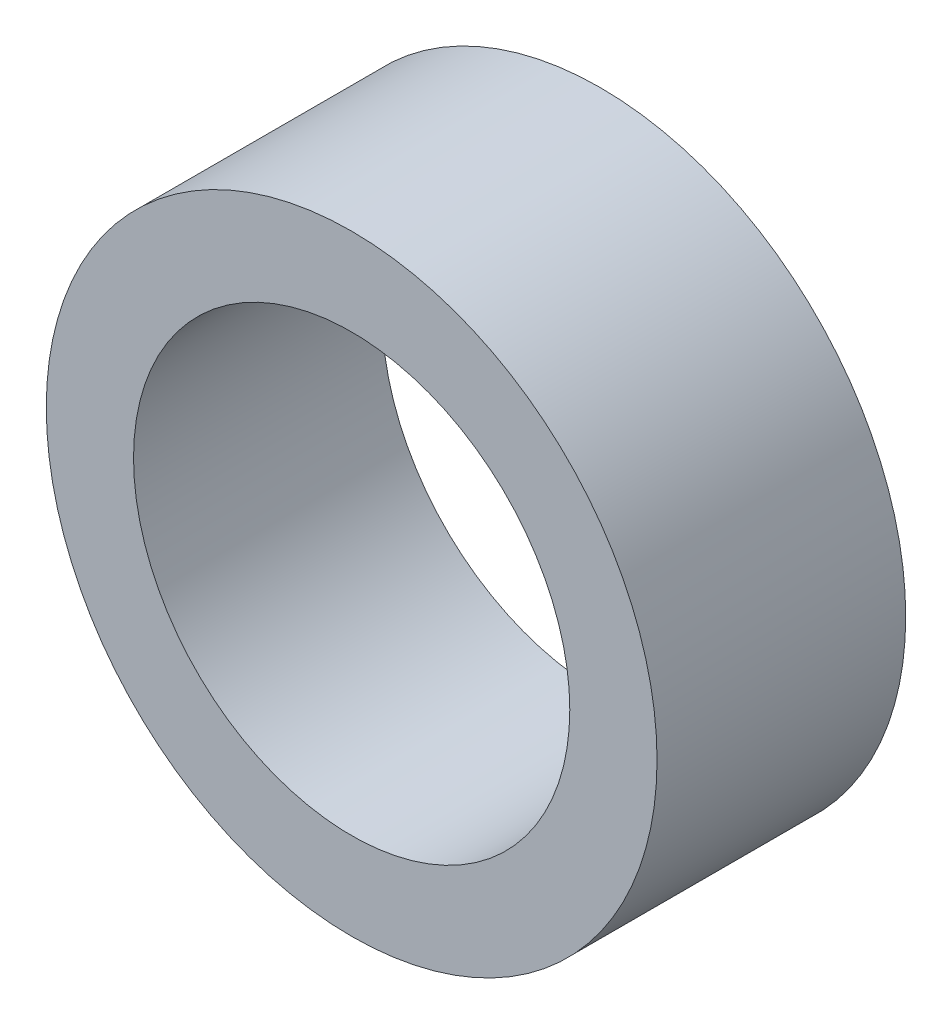
from build123d import *

# Parameters (mm, degrees)
SKETCH_1_R      = 7
SKETCH_1_R_2    = 5
EXTRUDE_1_DEPTH = 5.7


with BuildPart() as part:
    # 草图1 → 凸台-拉伸1 (new body)
    with BuildSketch(Plane.XY):
        Circle(SKETCH_1_R)
        Circle(SKETCH_1_R_2, mode=Mode.SUBTRACT)
    extrude(amount=EXTRUDE_1_DEPTH)


solid = part.part
